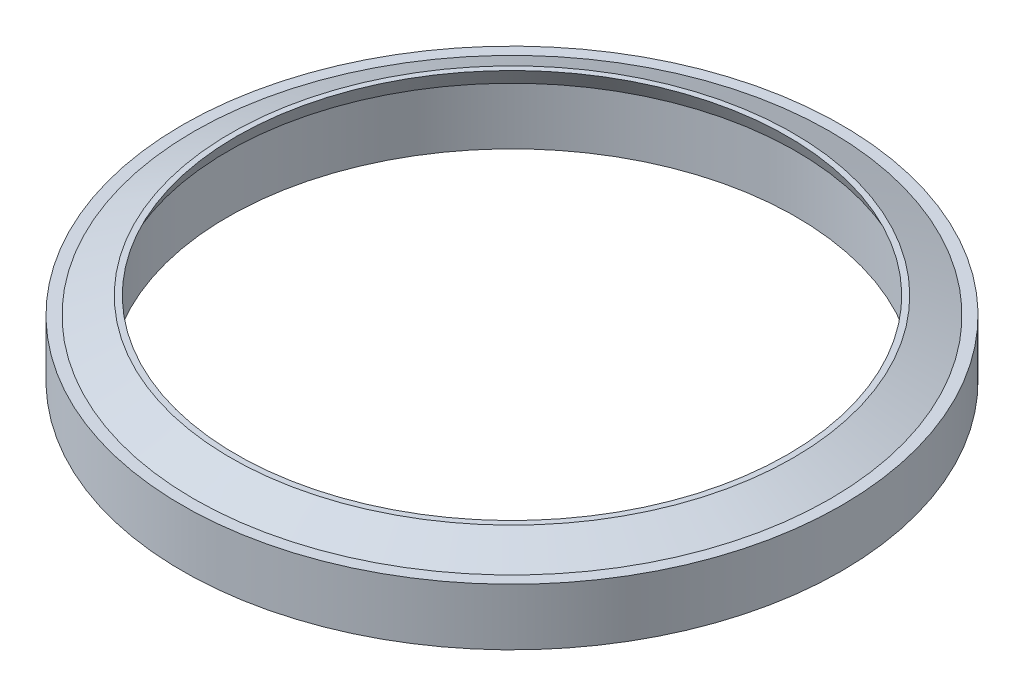
SolidWorks part; units mm, degrees
material "6061-T6 (SS)"
ref_plane "Front" through (0, 0, 0) normal (0, 0, 1) x (1, 0, 0)
ref_plane "Top" through (0, 0, 0) normal (0, 1, 0) x (1, 0, 0)
ref_plane "Right" through (0, 0, 0) normal (1, 0, 0) x (0, 0, -1)
sketch "Sketch2" plane through (0, 0, 0) normal (0, 0, 1) x (1, 0, 0)
  line L0 (0, -1000) -> (0, 49000) construction
  line L1 (25, 0) -> (29, 0)
  line L2 (29, 0) -> (29, 5)
  line L3 (29, 5) -> (28, 5)
  line L4 (28, 5) -> (24.75, 6.5)
  line L5 (24.75, 6.5) -> (24.25, 6.5)
  line L6 (24.25, 6.5) -> (25, 5)
  line L7 (25, 5) -> (25, 0)
  dimension "D1" = 50
  dimension "D2" = 58
  dimension "D3" = 5
  dimension "D4" = 0.5
  dimension "D5" = 6.5
  dimension "D6" = 48.5
  dimension "D7" = 56
revolve "Revolve1" add sketch "Sketch2" angle 360 about L0
